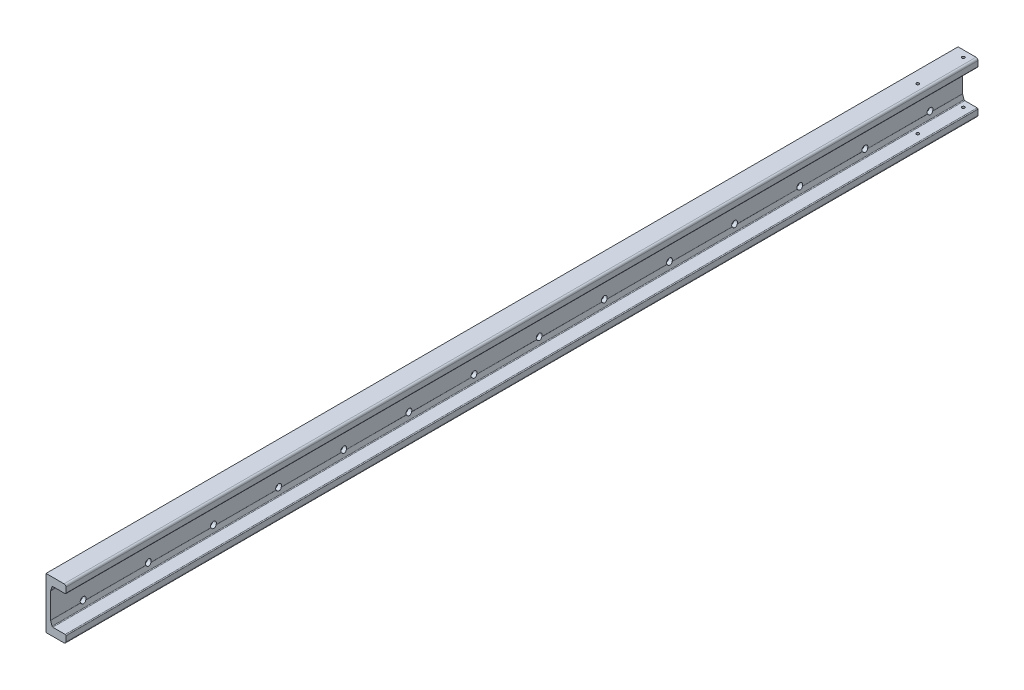
SolidWorks part; units mm, degrees
material "1023 碳钢板 (SS)"
ref_plane "前视基准面" through (0, 0, 0) normal (0, 0, 1) x (1, 0, 0)
ref_plane "上视基准面" through (0, 0, 0) normal (0, 1, 0) x (1, 0, 0)
ref_plane "右视基准面" through (0, 0, 0) normal (1, 0, 0) x (0, 0, -1)
sketch "草图1" plane through (0, 0, 0) normal (0, 0, 1) x (1, 0, 0)
  line L0 (0, 0) -> (-61.2, 0)
  line L1 (-61.2, 0) -> (-61.2, -157.2)
  line L2 (-61.2, -157.2) -> (0, -157.2)
  line L3 (0, -157.2) -> (0, -132.8)
  line L4 (0, -132.8) -> (-42.2, -132.8)
  line L5 (-47.2, -117.8) -> (-47.2, -39.4)
  line L6 (-42.2, -24.4) -> (0, -24.4)
  line L7 (0, -24.4) -> (0, 0)
  line L8 (-47.2, -117.8) -> (-42.2, -132.8)
  line L9 (-61.2, -78.6) -> (-16.126, -78.6) construction
  line L10 (-47.2, -39.4) -> (-42.2, -24.4)
  dimension "D1" = 157.2
  dimension "D2" = 24.4
  dimension "D3" = 108.4
  dimension "D4" = 61.2
  dimension "D5" = 14
  dimension "D6" = 15
extrude "凸台-拉伸1" add sketch "草图1" along normal blind 2800 contours L6 L7 L0 L1 L2 L3 L4 L8 L5 L10
fillet "圆角1" radius 6 2 edges at (0, -157.2, 1400) (0, 0, 1400)
fillet "圆角2" radius 2.5 6 edges at (-42.2, -132.8, 1400) (-47.2, -117.8, 1400) (-47.2, -39.4, 1400) (-42.2, -24.4, 1400) (0, -132.8, 1400) (0, -24.4, 1400)
sketch "草图2" plane through (-61.2, 0, 0) normal (-1, 0, 0) x (0, 0, 1)
  line L0 (0, 0) -> (0, -157.2) construction
  circle A0 centre (100, -113.6) radius 5.5
  circle A1 centre (100, -43.6) radius 5.5
  circle A2 centre (300, -43.6) radius 5.5
  circle A3 centre (300, -113.6) radius 5.5
  circle A4 centre (500, -43.6) radius 5.5
  circle A5 centre (500, -113.6) radius 5.5
  circle A6 centre (700, -43.6) radius 5.5
  circle A7 centre (700, -113.6) radius 5.5
  circle A8 centre (900, -43.6) radius 5.5
  circle A9 centre (900, -113.6) radius 5.5
  circle A10 centre (1100, -43.6) radius 5.5
  circle A11 centre (1100, -113.6) radius 5.5
  circle A12 centre (1300, -43.6) radius 5.5
  circle A13 centre (1300, -113.6) radius 5.5
  circle A14 centre (1500, -43.6) radius 5.5
  circle A15 centre (1500, -113.6) radius 5.5
  circle A16 centre (1700, -43.6) radius 5.5
  circle A17 centre (1700, -113.6) radius 5.5
  circle A18 centre (1900, -43.6) radius 5.5
  circle A19 centre (1900, -113.6) radius 5.5
  circle A20 centre (2100, -43.6) radius 5.5
  circle A21 centre (2100, -113.6) radius 5.5
  circle A22 centre (2300, -43.6) radius 5.5
  circle A23 centre (2300, -113.6) radius 5.5
  circle A24 centre (2500, -43.6) radius 5.5
  circle A25 centre (2500, -113.6) radius 5.5
  circle A26 centre (2700, -43.6) radius 5.5
  circle A27 centre (2700, -113.6) radius 5.5
  point P7 (0, -78.6)
  dimension "D1" = 11
  dimension "D2" = 11
  dimension "D3" = 100
  dimension "D5" = 35
  dimension "D6" = 14
  dimension "D4" = 70
extrude "切除-拉伸1" cut sketch "草图2" against normal blind 3
sketch "草图3" plane through (-58.2, 0, 0) normal (-1, 0, 0) x (0, 0, 1)
  circle A0 centre (100, -43.6) radius 9
  circle A1 centre (100, -113.6) radius 9
  circle A2 centre (300, -43.6) radius 9
  circle A3 centre (300, -113.6) radius 9
  circle A4 centre (500, -43.6) radius 9
  circle A5 centre (500, -113.6) radius 9
  circle A6 centre (700, -43.6) radius 9
  circle A7 centre (700, -113.6) radius 9
  circle A8 centre (900, -43.6) radius 9
  circle A9 centre (900, -113.6) radius 9
  circle A10 centre (1100, -43.6) radius 9
  circle A11 centre (1100, -113.6) radius 9
  circle A12 centre (1300, -43.6) radius 9
  circle A13 centre (1300, -113.6) radius 9
  circle A14 centre (1500, -43.6) radius 9
  circle A15 centre (1500, -113.6) radius 9
  circle A16 centre (1700, -43.6) radius 9
  circle A17 centre (1700, -113.6) radius 9
  circle A18 centre (1900, -43.6) radius 9
  circle A19 centre (1900, -113.6) radius 9
  circle A20 centre (2100, -43.6) radius 9
  circle A21 centre (2100, -113.6) radius 9
  circle A22 centre (2300, -43.6) radius 9
  circle A23 centre (2300, -113.6) radius 9
  circle A24 centre (2500, -43.6) radius 9
  circle A25 centre (2500, -113.6) radius 9
  circle A26 centre (2700, -43.6) radius 9
  circle A27 centre (2700, -113.6) radius 9
  dimension "D1" = 18
  dimension "D2" = 18
  dimension "D3" = 14
extrude "切除-拉伸2" cut sketch "草图3" against normal blind 31
sketch "草图4" plane through (0, 0, 0) normal (0, 1, 0) x (1, 0, 0)
  line L0 (0, 0) -> (0, -2800) construction
  line L1 (-6, 0) -> (-61.2, 0) construction
  circle A0 centre (-25, -20) radius 5
  circle A1 centre (-25, -160) radius 5
  point P4 (0, 0)
  dimension "D2" = 20
  dimension "D4" = 10
  dimension "D5" = 10
  dimension "D1" = 25
  dimension "D3" = 140
hole_wizard "M10 螺纹孔1" positions "草图5" profile "草图6" tap size "M10" standard "ISO" end condition through all
sketch "草图5" plane through (0, 0, 0) normal (0, 1, 0) x (1, 0, 0)
  point P0 (-25, -20)
  point P3 (-25, -160)
sketch "草图6" plane through (-25, 0, 20) normal (1, 0, 0) x (0, 0, 1)
  line L0 (0, 0) -> (0, 157.2)
  line L1 (0, 157.2) -> (4.25, 157.2)
  line L2 (4.25, 157.2) -> (4.25, 0)
  line L5 (4.25, 0) -> (0, 0)
  line L11 (0, -6.35) -> (0, 107.95) construction
  dimension "通孔螺纹孔钻头直径" = 8.5
  dimension "通孔螺纹孔钻头深度" = 157.2
cosmetic thread "孔螺蚊线1" parameters "D2"=10
cosmetic thread "孔螺蚊线2" parameters "D2"=10
